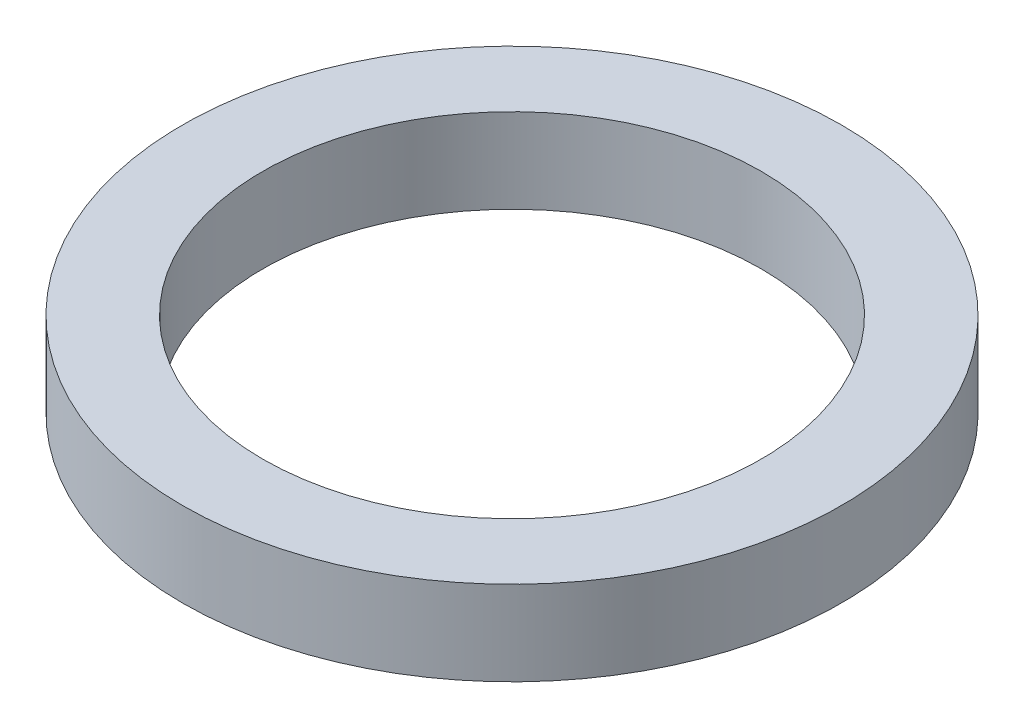
SolidWorks part; units mm, degrees
material "ABS"
ref_plane "Front Plane" through (0, 0, 0) normal (0, 0, 1) x (1, 0, 0)
ref_plane "Top Plane" through (0, 0, 0) normal (0, 1, 0) x (1, 0, 0)
ref_plane "Right Plane" through (0, 0, 0) normal (1, 0, 0) x (0, 0, -1)
sketch "Sketch1" plane through (0, 0, 0) normal (0, 1, 0) x (1, 0, 0)
  circle A0 centre (0, 0) radius 7.8
  circle A1 centre (0, 0) radius 5.9
  dimension "D1" = 15.6
  dimension "D2" = 1.9
extrude "Boss-Extrude1" add sketch "Sketch1" along normal blind 2
